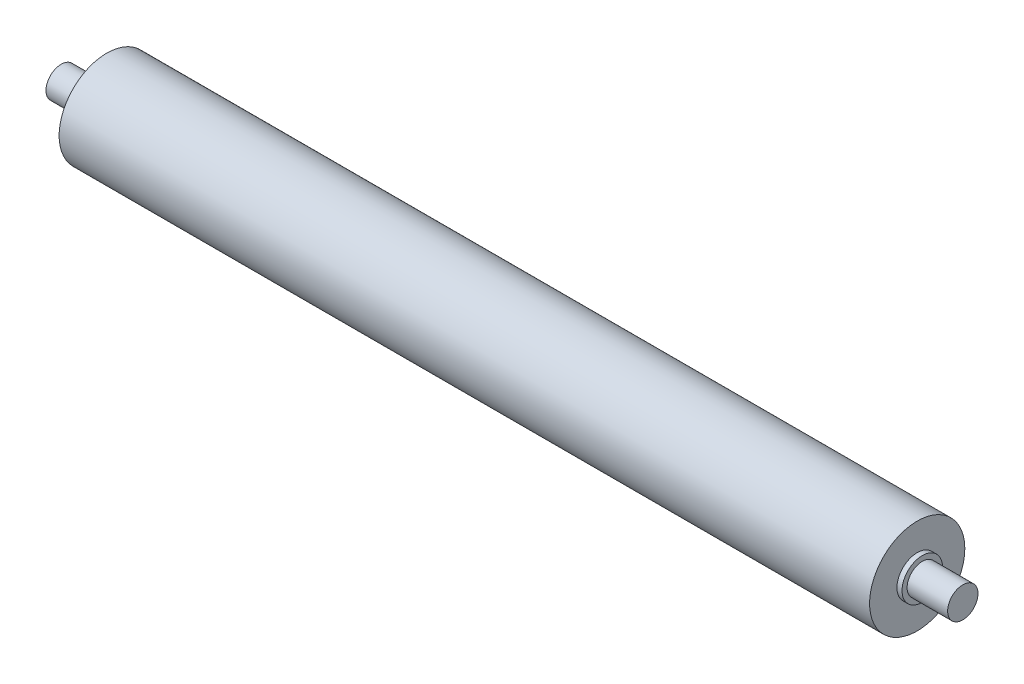
from build123d import *


with BuildPart() as part:
    # Sketch1 → Revolve1 (revolve)
    with BuildSketch(Plane.XY, mode=Mode.PRIVATE) as revolve1_sk:
        Polygon((0, 0), (0, 7.5), (20, 7.5), (20, 10), (22.5, 10), (22.5, 23.5), (422.5, 23.5), (422.5, 10), (425, 10), (425, 7.5), (445, 7.5), (445, 0), align=None)
    revolve(revolve1_sk.sketch.rotate(Axis((0, 0, 0), (-1, 0, 0)), 90), axis=Axis((0, 0, 0), (-1, 0, 0)))


solid = part.part
